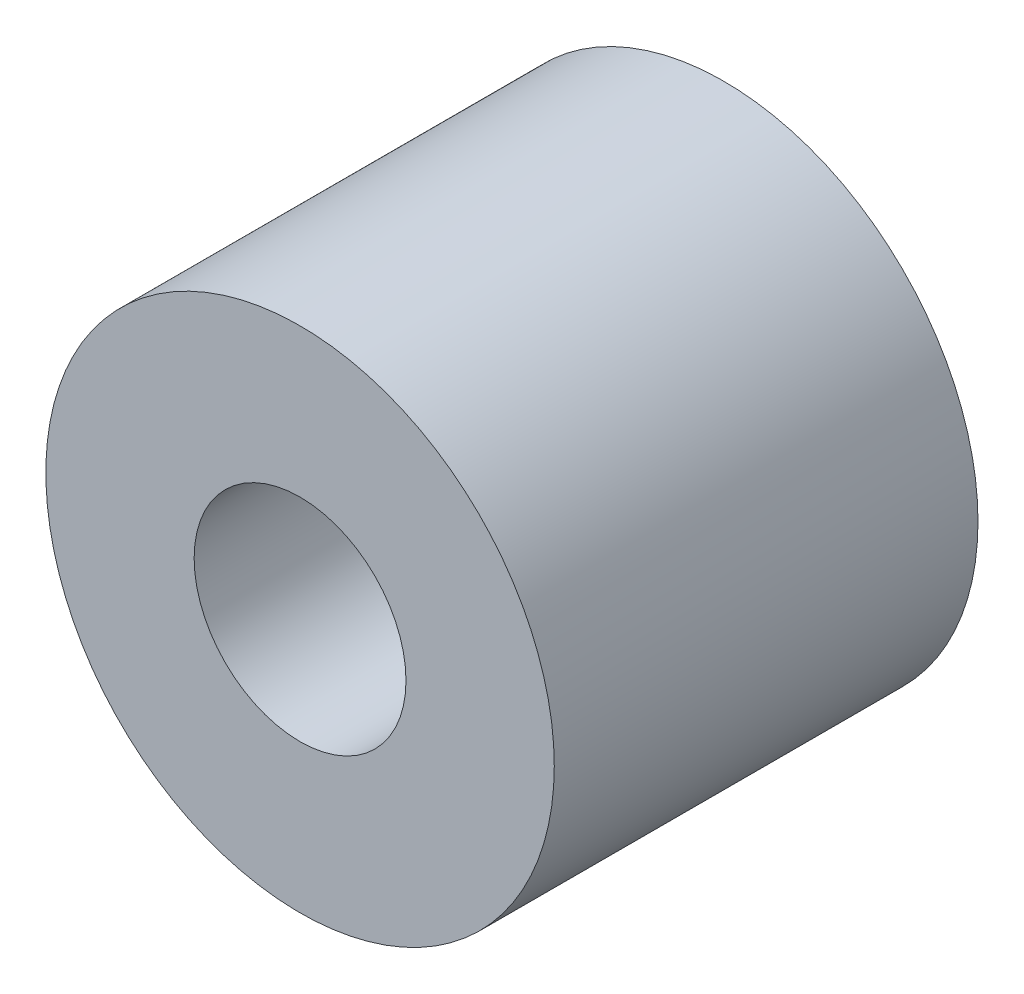
SolidWorks part; units mm, degrees
ref_plane "Front Plane" through (0, 0, 0) normal (0, 0, 1) x (1, 0, 0)
ref_plane "Top Plane" through (0, 0, 0) normal (0, 1, 0) x (1, 0, 0)
ref_plane "Right Plane" through (0, 0, 0) normal (1, 0, 0) x (0, 0, -1)
sketch "Sketch1" plane through (0, 0, 0) normal (0, 0, 1) x (1, 0, 0)
  circle A0 centre (0, 0) radius 84
  circle A1 centre (0, 0) radius 35
  dimension "D1" = 168
  dimension "D2" = 70
extrude "Boss-Extrude1" add sketch "Sketch1" along normal mid plane 140
